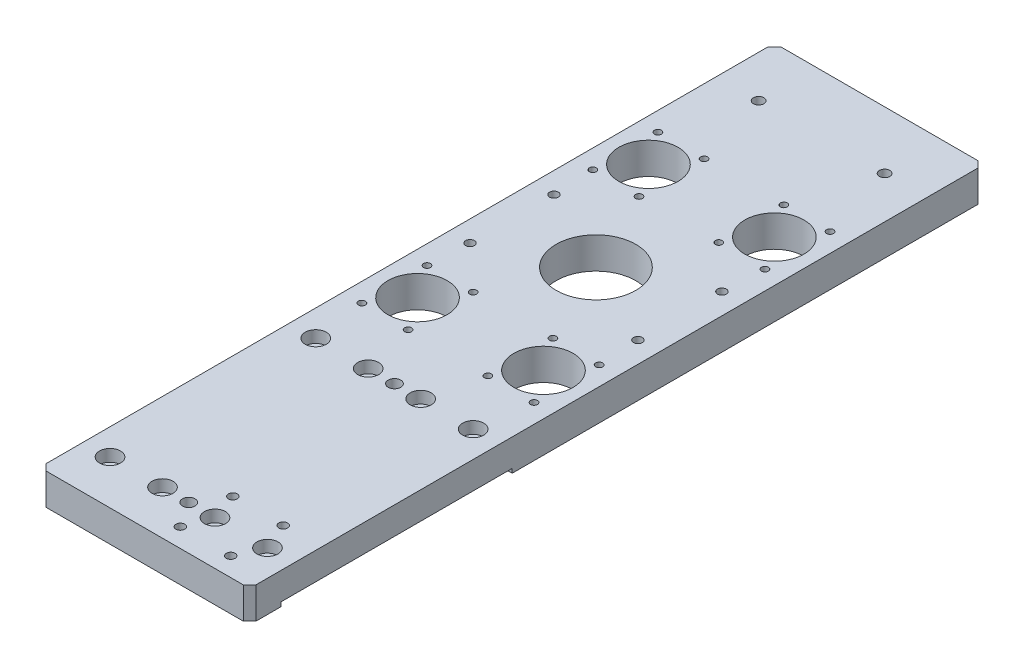
from build123d import *

# Parameters (mm, degrees)
SKETCH_1_W                = 100
SKETCH_1_H                = 350
EXTRUDE_1_DEPTH           = 15
SKETCH_3_W                = 100
SKETCH_3_H                = 110.2
CUT_EXTRUDE_1_DEPTH       = 2
HOLE_WIZARD_1_D           = 5.5
HOLE_WIZARD_1_DEPTH       = 15
HOLE_WIZARD_1_CBORE_D     = 10
HOLE_WIZARD_1_CBORE_DEPTH = 5.7
HOLE_WIZARD_1_TIP         = 1.652366702
MM_1_D                    = 6
MM_1_DEPTH                = 15
MM_1_TIP                  = 1.802581857
SKETCH_8_R                = 19
CUT_EXTRUDE_2_DEPTH       = 20
CHAMFER_1_SIZE            = 3
SKETCH_9_R                = 14.1
CUT_EXTRUDE_3_DEPTH       = 20
MM_2_D                    = 5
MM_2_DEPTH                = 20
MM_2_TIP                  = 1.502151548
HOLE_WIZARD_M5_1_D        = 4.2
HOLE_WIZARD_M5_1_DEPTH    = 20
HOLE_WIZARD_M5_1_TIP      = 1.2618073
HOLE_WIZARD_M4_1_D        = 3.3
HOLE_WIZARD_M4_1_DEPTH    = 32
HOLE_WIZARD_M4_1_TIP      = 0.991420021
HOLE_WIZARD_M5_2_D        = 4.2
HOLE_WIZARD_M5_2_DEPTH    = 20
HOLE_WIZARD_M5_2_TIP      = 1.2618073


with BuildPart() as part:
    # 草图1 → 凸台-拉伸1 (new body)
    with BuildSketch(Plane(origin=(0, 0, 0), x_dir=(1, 0, 0), z_dir=(0, 1, 0))):
        Rectangle(SKETCH_1_W, SKETCH_1_H)
    extrude(amount=EXTRUDE_1_DEPTH)

    # 草图3 → 切除-拉伸1 (cut)
    with BuildSketch(Plane.XZ):
        with Locations((0, 105)):
            Rectangle(SKETCH_3_W, SKETCH_3_H)
    extrude(amount=-CUT_EXTRUDE_1_DEPTH, mode=Mode.SUBTRACT)

    # 打孔尺寸(%根据)内六角圆柱头螺钉的类型1
    with Locations(Plane(origin=(0, 15, 0), x_dir=(1, 0, 0), z_dir=(0, 1, 0))):
        with Locations((-37.5, -154), (-12.5, -154), (12.5, -154), (37.5, -154), (-37.5, -56), (-12.5, -56), (12.5, -56), (37.5, -56)):
            CounterBoreHole(HOLE_WIZARD_1_D / 2, HOLE_WIZARD_1_CBORE_D / 2, HOLE_WIZARD_1_CBORE_DEPTH, depth=HOLE_WIZARD_1_DEPTH)
            with Locations((0, 0, -(HOLE_WIZARD_1_DEPTH + HOLE_WIZARD_1_TIP / 2))):  # 118° drill point
                Cone(0, HOLE_WIZARD_1_D / 2, HOLE_WIZARD_1_TIP, mode=Mode.SUBTRACT)

    # 大小mm 暗销孔1
    with Locations(Plane(origin=(0, 15, 0), x_dir=(1, 0, 0), z_dir=(0, 1, 0))):
        with Locations((0, -154), (0, -56)):
            Hole(MM_1_D / 2, depth=MM_1_DEPTH)
            with Locations((0, 0, -(MM_1_DEPTH + MM_1_TIP / 2))):  # 118° drill point
                Cone(0, MM_1_D / 2, MM_1_TIP, mode=Mode.SUBTRACT)

    # 草图8 → 切除-拉伸2 (cut)
    with BuildSketch(Plane(origin=(0, 15, 0), x_dir=(1, 0, 0), z_dir=(0, 1, 0))):
        with Locations(Location((0, 40, 0), (0, 0, 270))):
            Circle(SKETCH_8_R)
    extrude(amount=-CUT_EXTRUDE_2_DEPTH, mode=Mode.SUBTRACT)

    # 倒角1
    chamfer_1_edges = [part.edges().sort_by_distance(p)[0] for p in [
        (50, 7.5, 175),
        (-50, 7.5, 175),
        (-50, 7.5, -175),
        (50, 7.5, -175),
    ]]
    chamfer(chamfer_1_edges, length=CHAMFER_1_SIZE)

    # 草图9 → 切除-拉伸3 (cut)
    with BuildSketch(Plane(origin=(0, 15, 0), x_dir=(1, 0, 0), z_dir=(0, 1, 0))):
        with Locations(Location((30, -15, 0), (0, 0, 270))):
            Circle(SKETCH_9_R)
        with Locations(Location((30, 95, 0), (0, 0, 270))):
            Circle(SKETCH_9_R)
        with Locations(Location((-30, -15, 0), (0, 0, 270))):
            Circle(SKETCH_9_R)
        with Locations(Location((-30, 95, 0), (0, 0, 270))):
            Circle(SKETCH_9_R)
    extrude(amount=-CUT_EXTRUDE_3_DEPTH, mode=Mode.SUBTRACT)

    # 大小mm 暗销孔2
    with Locations(Plane(origin=(0, 15, 0), x_dir=(1, 0, 0), z_dir=(0, 1, 0))):
        with Locations((29.999999986, 147.499999994), (-30.000000014, 147.499999994)):
            Hole(MM_2_D / 2, depth=MM_2_DEPTH)
            with Locations((0, 0, -(MM_2_DEPTH + MM_2_TIP / 2))):  # 118° drill point
                Cone(0, MM_2_D / 2, MM_2_TIP, mode=Mode.SUBTRACT)

    # M5 螺纹孔1
    with Locations(Plane(origin=(0, 0, 0), x_dir=(-1, 0, 0), z_dir=(0, -1, 0))):
        with Locations((40, 19.999999999), (-40, 19.999999999), (40, 59.999999999), (-40, 59.999999999)):
            Hole(HOLE_WIZARD_M5_1_D / 2, depth=HOLE_WIZARD_M5_1_DEPTH)
            with Locations((0, 0, -(HOLE_WIZARD_M5_1_DEPTH + HOLE_WIZARD_M5_1_TIP / 2))):  # 118° drill point
                Cone(0, HOLE_WIZARD_M5_1_D / 2, HOLE_WIZARD_M5_1_TIP, mode=Mode.SUBTRACT)

    # M4 螺纹孔1
    with Locations(Plane(origin=(0, 15, 0), x_dir=(1, 0, 0), z_dir=(0, 1, 0))):
        with Locations((41, -30.5), (19, -30.5), (41, 0.5), (19, 0.5), (-19, -30.5), (-41, -30.5), (-19, 0.5), (-41, 0.5), (41, 79.5), (19, 79.5), (41, 110.5), (19, 110.5), (-19, 79.5), (-41, 79.5), (-19, 110.5), (-41, 110.5)):
            Hole(HOLE_WIZARD_M4_1_D / 2, depth=HOLE_WIZARD_M4_1_DEPTH)
            with Locations((0, 0, -(HOLE_WIZARD_M4_1_DEPTH + HOLE_WIZARD_M4_1_TIP / 2))):  # 118° drill point
                Cone(0, HOLE_WIZARD_M4_1_D / 2, HOLE_WIZARD_M4_1_TIP, mode=Mode.SUBTRACT)

    # M5 螺纹孔2
    with Locations(Plane(origin=(0, 15, 0), x_dir=(1, 0, 0), z_dir=(0, 1, 0))):
        with Locations((8, -141), (32, -141), (8, -166), (32, -166)):
            Hole(HOLE_WIZARD_M5_2_D / 2, depth=HOLE_WIZARD_M5_2_DEPTH)
            with Locations((0, 0, -(HOLE_WIZARD_M5_2_DEPTH + HOLE_WIZARD_M5_2_TIP / 2))):  # 118° drill point
                Cone(0, HOLE_WIZARD_M5_2_D / 2, HOLE_WIZARD_M5_2_TIP, mode=Mode.SUBTRACT)


solid = part.part
